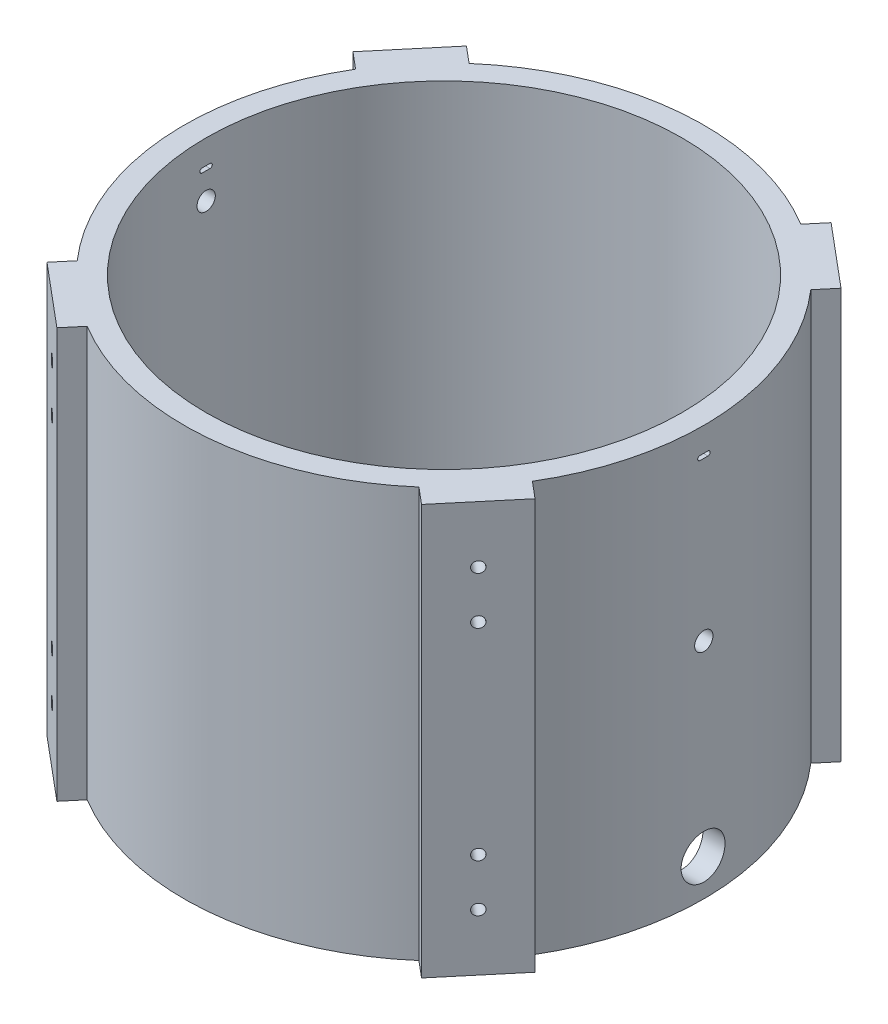
from build123d import *

# Parameters (mm, degrees)
SKETCH1_W                = 6
SKETCH1_H                = 112
CUT_EXTRUDE1_DEPTH       = 10
SKETCH3_R                = 6
CUT_EXTRUDE2_DEPTH       = 10
CUT_EXTRUDE5_DEPTH       = 195.291019003
CUT_EXTRUDE5_DEPTH_BACK  = 195.291019003
SKETCH_5_4_R             = 2.5
CUT_EXTRUDE6_DEPTH       = 300
BOSS_EXTRUDE3_START      = 71
SKETCH10_W               = 112
SKETCH10_H               = 22
BOSS_EXTRUDE3_DEPTH      = 5
SKETCH12_R               = 1.5
CUT_EXTRUDE10_DEPTH      = 5
CIRPATTERN14_COUNT       = 4
CUT_EXTRUDE12_REACH      = 152.419
CUT_EXTRUDE12_END_RADIUS = 71
SKETCH_5_4_2_R           = 2.5


with BuildPart() as part:
    # Sketch1 → Revolve1 (revolve)
    with BuildSketch(Plane.XY, mode=Mode.PRIVATE) as revolve1_sk:
        with Locations((68, 56)):
            Rectangle(SKETCH1_W, SKETCH1_H)
    revolve(revolve1_sk.sketch.rotate(Axis((0, -61.12033846, 0), (0, 1, 0)), 90), axis=Axis((0, -61.12033846, 0), (0, 1, 0)))

    # Sketch2 → Cut-Extrude1 (cut)
    with BuildSketch(Plane(origin=(71, 0, 0), x_dir=(0, 0, -1), z_dir=(1, 0, 0))):
        with BuildLine():
            Line((-1.1, 105.4), (1.1, 105.4))
            ThreePointArc((1.1, 105.4), (1.7, 104.8), (1.1, 104.2))
            Line((1.1, 104.2), (-1.1, 104.2))
            ThreePointArc((-1.1, 104.2), (-1.7, 104.8), (-1.1, 105.4))
        make_face()
    extrude(amount=-CUT_EXTRUDE1_DEPTH, mode=Mode.SUBTRACT)

    # Sketch3 → Cut-Extrude2 (cut)
    with BuildSketch(Plane(origin=(71, 0, 0), x_dir=(0, 0, -1), z_dir=(1, 0, 0))):
        with Locations((0, 10)):
            Circle(SKETCH3_R)
    extrude(amount=-CUT_EXTRUDE2_DEPTH, mode=Mode.SUBTRACT)

    # Sketch4 → Cut-Extrude5 (cut, two sides: drawn at the far end of the back side and taken through both)
    with BuildSketch(Plane(origin=(-71, 0, 0), x_dir=(0, 0, -1), z_dir=(1, 0, 0)).offset(-CUT_EXTRUDE5_DEPTH_BACK)):
        with BuildLine():
            Line((-1.1, 105.4), (1.1, 105.4))
            ThreePointArc((1.1, 105.4), (1.7, 104.8), (1.1, 104.2))
            Line((1.1, 104.2), (-1.1, 104.2))
            ThreePointArc((-1.1, 104.2), (-1.7, 104.8), (-1.1, 105.4))
        make_face()
    extrude(amount=CUT_EXTRUDE5_DEPTH + CUT_EXTRUDE5_DEPTH_BACK, mode=Mode.SUBTRACT)

    # Sketch 5_4 → Cut-Extrude6 (cut)
    with BuildSketch(Plane(origin=(0, 0, 0), x_dir=(0, 0, -1), z_dir=(1, 0, 0))):
        with Locations((0, 97.06)):
            Circle(SKETCH_5_4_R)
    extrude(amount=-CUT_EXTRUDE6_DEPTH, mode=Mode.SUBTRACT)

    # Sketch10 → Boss-Extrude3 (add, symmetric)
    with BuildSketch(Plane(origin=(0, 0, 0), x_dir=(0, -1, 0), z_dir=(-0.7660444431189771, 0, -0.6427876096865406)).offset(BOSS_EXTRUDE3_START)):
        with Locations((-56, 0)):
            Rectangle(SKETCH10_W, SKETCH10_H)
    boss_extrude3 = extrude(amount=BOSS_EXTRUDE3_DEPTH, both=True)

    # Sketch12 → Cut-Extrude10 (cut)
    with BuildSketch(Plane(origin=(-58.219377677, 0, -48.851858336), x_dir=(-0.6427876096865407, 0, 0.766044443118977), z_dir=(-0.766044443118977, 0, -0.6427876096865407))):
        with Locations((0, 96.5)):
            Circle(SKETCH12_R)
        with Locations((0, 83.5)):
            Circle(SKETCH12_R)
        with Locations(Location((0, 28.5, 0), (0, 0, 180))):
            Circle(SKETCH12_R)
        with Locations(Location((0, 15.5, 0), (0, 0, 180))):
            Circle(SKETCH12_R)
    cut_extrude10 = extrude(amount=-CUT_EXTRUDE10_DEPTH, mode=Mode.SUBTRACT)

    # CirPattern14: Boss-Extrude3, Cut-Extrude10 ×4 about axis
    cirpattern14_axis = Axis((0, 0, 0), (0, 1, 0))
    add([boss_extrude3.rotate(cirpattern14_axis, i * 360 / CIRPATTERN14_COUNT) for i in range(1, CIRPATTERN14_COUNT)])
    add([cut_extrude10.rotate(cirpattern14_axis, i * 360 / CIRPATTERN14_COUNT) for i in range(1, CIRPATTERN14_COUNT)], mode=Mode.SUBTRACT)

    # Cut-Extrude12: up to this cylinder (the profile starts inside it)
    cut_extrude12_end = Plane(origin=(0, 61, 0), z_dir=(0, -1, 0)) * Cylinder(CUT_EXTRUDE12_END_RADIUS, 447.838, mode=Mode.PRIVATE)
    # Sketch 5_4 2 → Cut-Extrude12 (cut, up to the surface)
    with BuildSketch(Plane(origin=(0, 0, 0), x_dir=(0, 0, -1), z_dir=(1, 0, 0)), mode=Mode.PRIVATE) as cut_extrude12_sk1:
        with Locations(Location((0, 61, 0), (0, 0, 180))):
            Circle(SKETCH_5_4_2_R)
    cut_extrude12_tool1 = extrude(cut_extrude12_sk1.sketch, amount=CUT_EXTRUDE12_REACH, mode=Mode.PRIVATE) & cut_extrude12_end
    add(cut_extrude12_tool1.solids().sort_by_distance((0, 61, 0))[0], mode=Mode.SUBTRACT)


solid = part.part
